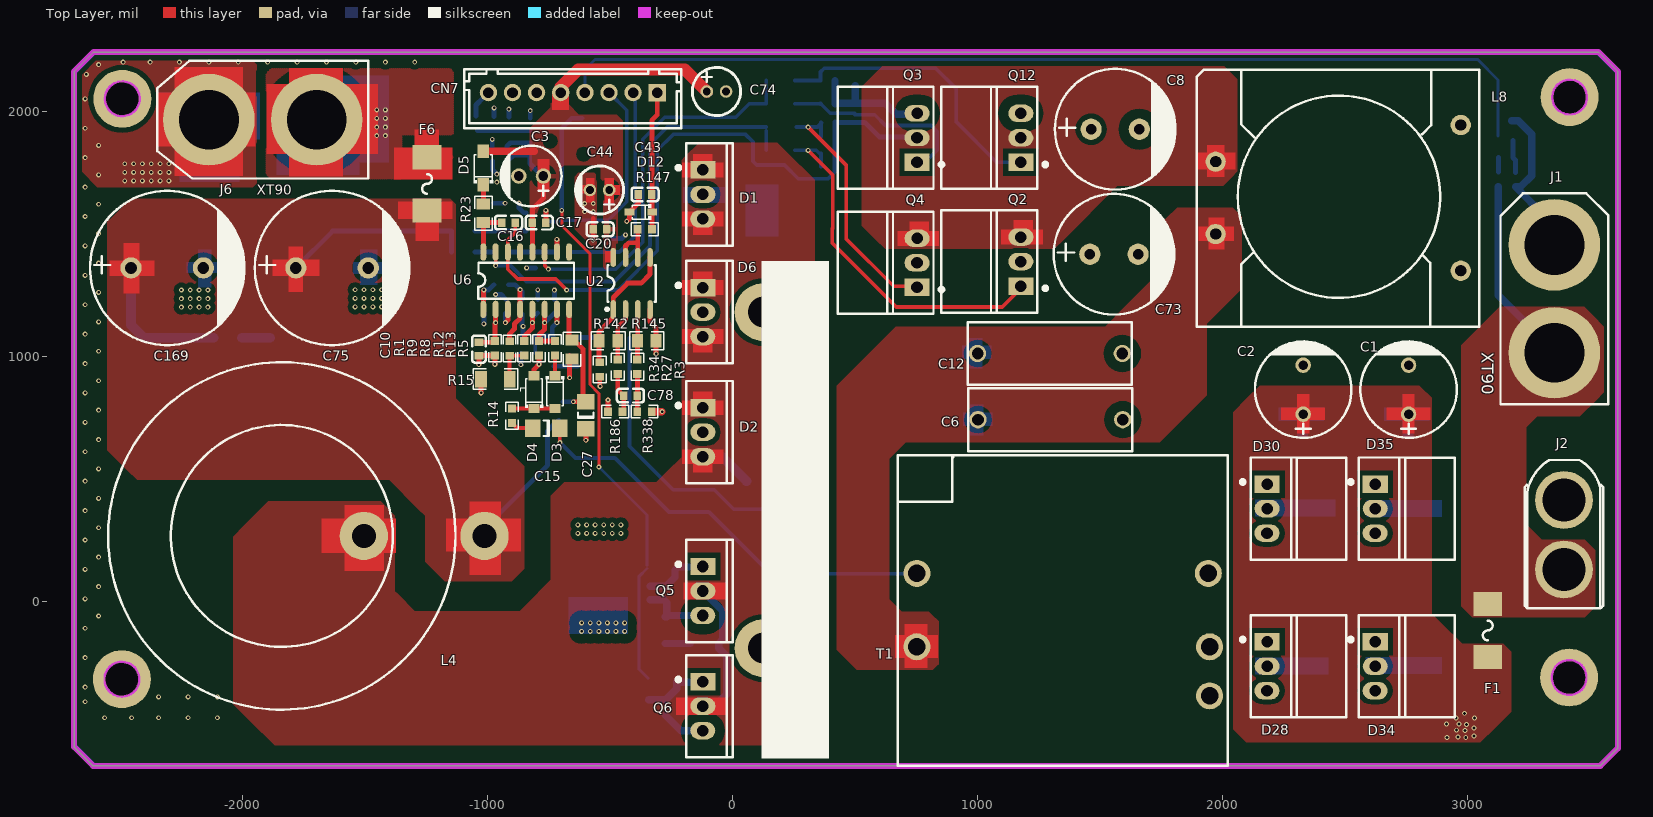
[diagram p0: Top Layer view]
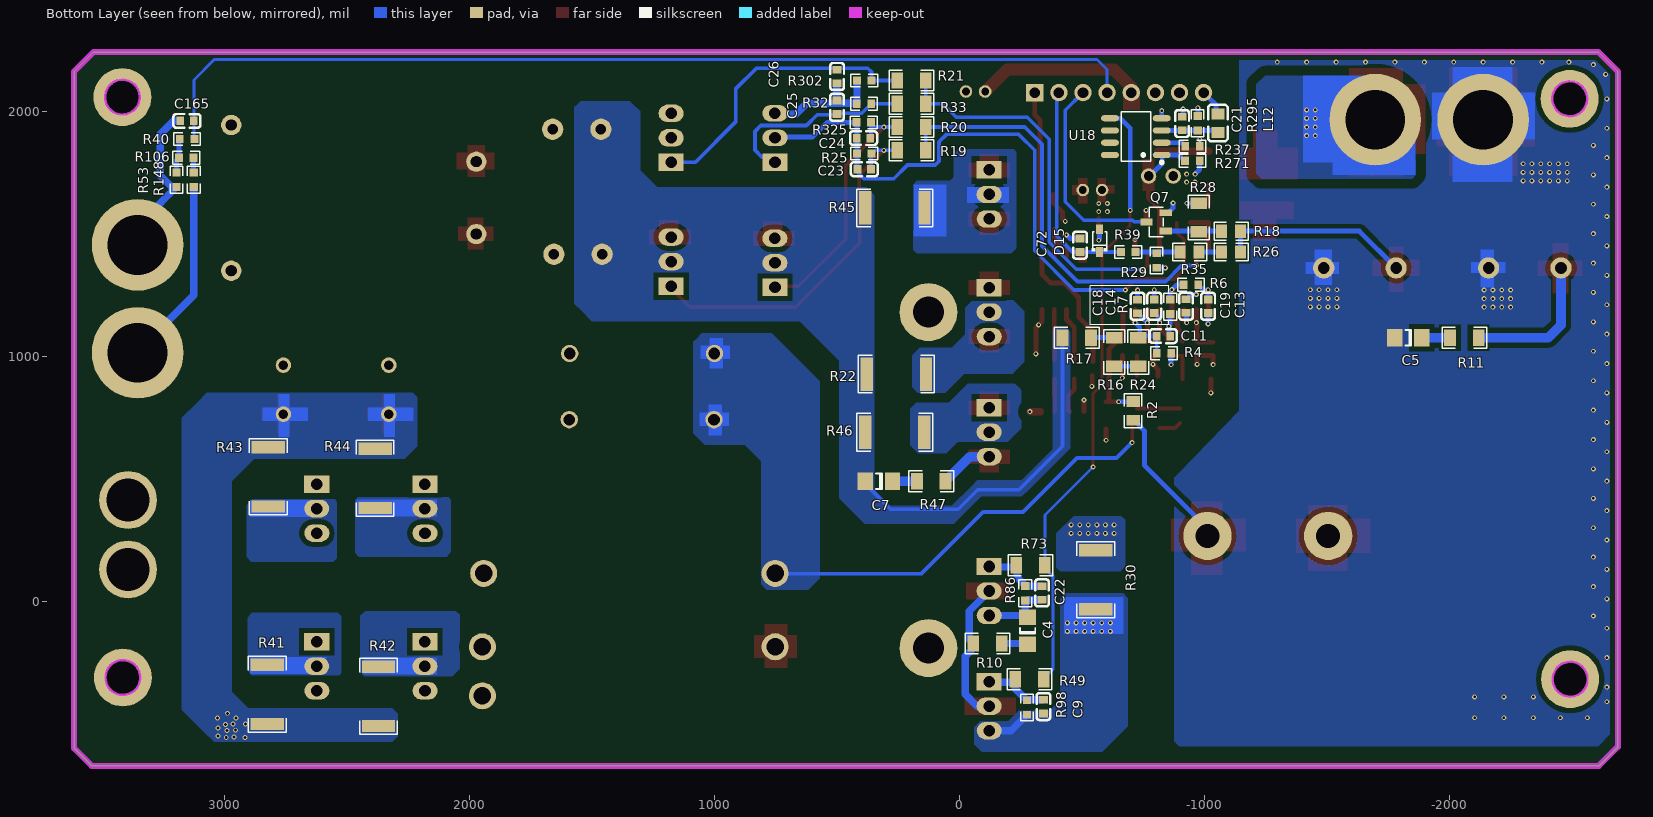
[diagram p1: Bottom Layer view, seen from below]
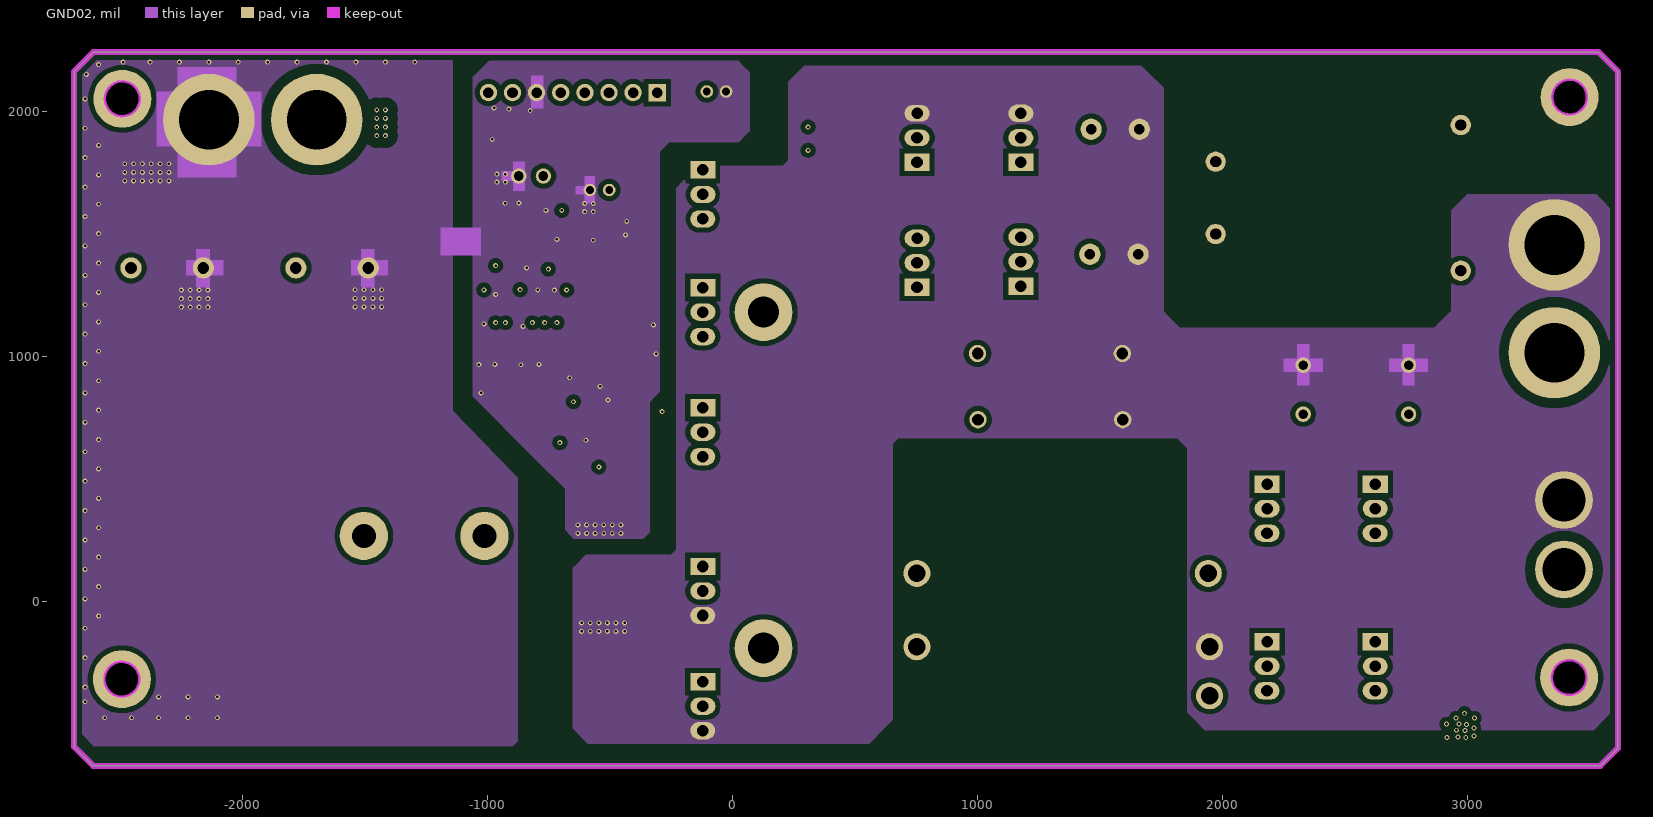
[diagram p2: GND02]
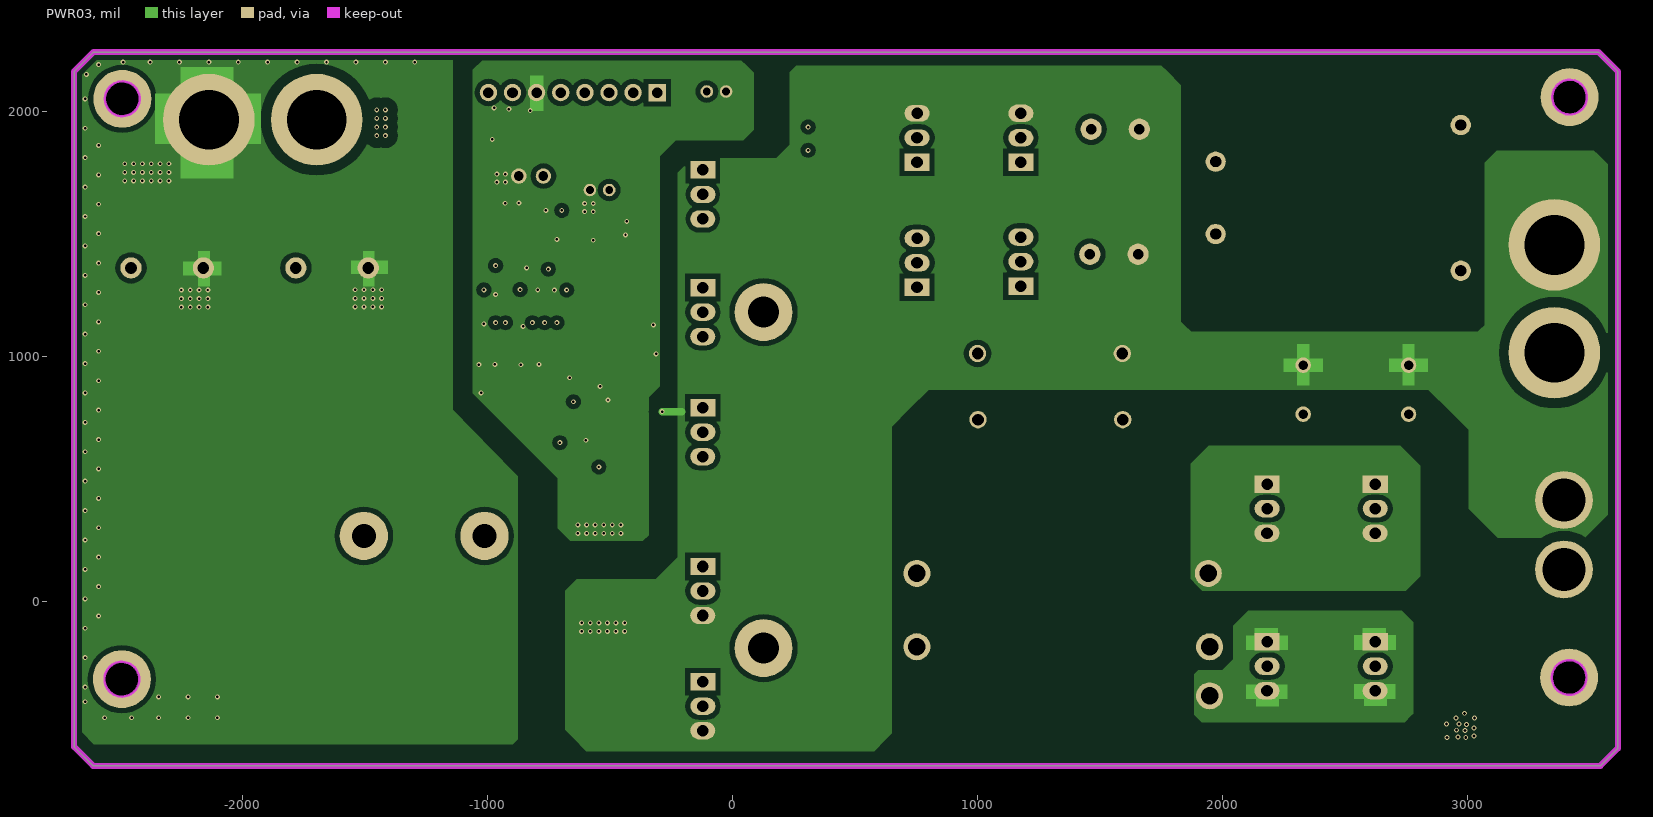
[diagram p3: PWR03]
# Altium PCB MISC89356.PcbDoc (part 1 of 3)
Units mil, origin at the board's own origin, x right, y up, seen from the top; angles counter-clockwise.
Board outline 6299.21 x 2912.91 mil, 4 copper layers (Top Layer, GND02, PWR03, Bottom Layer); 128 components, 68 nets, 313 pads, 200 vias.

## Layer stack, top to bottom (the 12.6 mil dielectric is the usual default, probably not edited)
Top Layer: signal copper 1.4
Dielectric: core 12.6, FR-4, Dk 4.8
GND02: signal copper 1.4
Dielectric: prepreg 12.6, FR-4, Dk 4.8
PWR03: signal copper 1.4
Dielectric: core 12.6, FR-4, Dk 4.8
Bottom Layer: signal copper 1.4

## Board outline
-2687.15,-592 -2609.15,-670 3539.85,-670 3612.07,-597.79 3612.07,2164.17 3533.33,2242.91 -2608.41,2242.91 -2687.15,2164.17

## Design rules (kind name [scope] priority, off if disabled: settings)
Clearance inpoly&Net [inpoly vs InNet('BAT-') or InNet('B+') or InNet('PV+')  or InNet('SW-PV') OR InNet('NETC75_1')] p1: gap=40
Clearance inpoly&inpoly [inpoly vs inpoly] p2: gap=20
Clearance INPOLY*All [INPOLY] p3: gap=20
Clearance Clearance_2 [isvia vs inpoly] p4: gap=10
Clearance Clearance_1 [All] p5: gap=8
ComponentClearance [All] p1 off: gap=10 collisioncheckmode=3 verticalgap=10 showdistances=FALSE
FabricationTestPointUsage TestPointUsage [All] p1: valid=0 allowmultiple=FALSE
FabricationTestpoint Testpoint [(IsPad And (OnTopLayer Or OnBottomLayer))] p1: side=3 testpointundercomponent=TRUE minsize=40 maxsize=100 preferedsize=60 minholesize=0 maxholesize=40 preferedholesize=32 testpointgrid=1 allowsidetop=TRUE allowsidebottom=TRUE usegrid=TRUE gridtolerance=0.01
Height [All] p1 off: minheight=0 maxheight=1000 prefheight=500
HoleSize [All] p1 off: absolutevalues=TRUE maxlimit=100 minlimit=1 maxpercent=80.000 minpercent=20.000
HoleToHoleClearance [All] p1 off: gap=10 allowstackedmicrovias=TRUE
LayerPairs [All] p1 off: enforce=TRUE
MinimumSolderMaskSliver [All] p1 off: minsoldermaskwidth=10
NetAntennae [All] p1: netantennaetolerance=1
PlaneClearance [All] p1: clearance=12
PlaneConnect [All] p1: planeconnectstyle=Relief reliefexpansion=8 reliefentries=4 reliefconductorwidth=10 reliefairgap=10
PolygonConnect PolygonConnect_1 [ISVIA] p1: connectstyle=Direct reliefconductorwidth=10 reliefentries=4 polygonreliefangle="90 Angle"
PolygonConnect [All] p2: connectstyle=Direct reliefconductorwidth=20 reliefentries=4 polygonreliefangle="90 Angle"
RoutingVias [All] p1: holewidth=10 width=20 viastyle="Through Hole" minholewidth=10 minwidth=20 maxholewidth=10 maxwidth=20
SilkToSilkClearance [All] p1 off: silktosilkclearance=10
SilkscreenOverComponentPads [IsPad] p1 off: minsilkscreentomaskgap=10
SolderMaskExpansion [All] p1: expansion=2.5
Width [All] p1: maxlimit=500 minlimit=10 preferedwidth=10
15 further rules are at their usual default settings.

## Components (designator, comment, footprint, x,y, rotation, side; value= is the part's Value field where it differs from the comment)
C1 "390uF" CAP-TH_BD10.0-P5.00-D1.0-FD 2757.85,867 r90 top
C2 "390uF" CAP-TH_BD10.0-P5.00-D1.0-FD 2327.85,867 r90 top
C3 "220uF" CAP-TH_BD6.3-P2.50-D1.0-FD -822.54,1737 r180 top
C4 "2.2nF" C1206 -278.15,-118.12 r90 bottom
C5 "2.2nF" C1206 -1832.03,1077 r0 bottom
C6 "150nF" CAP-TH_L17.0-W6.5-P15.00-D1.2 1296.41,743 r0 top
C7 "2.2nF" C1206 327.97,492 r0 bottom
C8 "150uF" CAP-TH_BD12.5-P5.00-D0.6-FD 1560.85,1928 r0 top
C9 "2.2nF" C0603 -343,-427.85 r270 bottom
C10 "220nF" C0603 -1035.15,1031.25 r90 top
C11 "1uF" C0603 -832.59,1083.69 r180 bottom
C12 "150nF" CAP-TH_L17.0-W6.5-P15.00-D1.2 1294.56,1013 r0 top
C13 "2.2uF" C0603 -1015.15,1206.14 r90 bottom
C14 "2.2uF" C0603 -795.15,1206.14 r270 bottom
C15 "NC" C1206 -760.03,708.69 r180 top
C16 "100nF" C0603 -914.59,1547 r180 top
C17 "100nF" C0603 -789.59,1547 r180 top
C18 "470pF" C0603 -727.15,1205.25 r270 bottom
C19 "1nF" C0603 -925.15,1206.25 r90 bottom
C20 "100nF" C0603 -541.27,1520 r180 top
C21 "220pF" C0603 -908.85,1951 r270 bottom
C22 "2.2nF" C0603 -337.15,36 r270 bottom
C23 "2.2nF" C0603 388,1764.85 r0 bottom
C24 "2.2nF" C0603 391,1891.85 r0 bottom
C25 "2.2nF" C0603 499.15,2018 r90 bottom
C26 "2.2nF" C0603 498.85,2143 r270 bottom
C27 "10nF" C1206 -599.15,761 r90 top
C43 "1nF" C0603 -357.15,1662 r0 top
C44 "22uF" CAP-TH_BD5.0-P2.00-D0.8-FD -543.08,1680 r180 top
C72 "100nF" C0603 -492.15,1454.67 r270 bottom
C73 "150uF" CAP-TH_BD12.5-P5.00-D0.6-FD 1555.85,1418 r0 top
C74 "22uF" CAP-TH_BD5.0-P2.00-D0.8-FD -66.15,2082 r0 top
C75 "560uF" CAP-TH_BD16.0-P7.50-D1.2-FD -1634.49,1362 r0 top
C78 "100nF" C0603 -416.83,841.01 r0 top
C165 "100nF" C0603 3151.41,1962 r180 bottom
C169 "560uF" CAP-TH_BD16.0-P7.50-D1.2-FD -2307.15,1362 r0 top
CN7 "HX25003-8A" CONN-TH_8P-P2.50_HX25003-8A -652.15,2052 r0 top
D1 "SBD20C200T" TO-220-3_L10.0-W4.5-P2.54-L -112.15,1662 r270 top
D2 "SBD20C200T" TO-220-3_L10.0-W4.5-P2.54-L -112.15,692 r270 top
D3 "1N4148W_C388533" SOD-123_L2.8-W1.8-LS3.7-RD -725.15,855.32 r270 top
D4 "1N4148W_C388533" SOD-123_L2.8-W1.8-LS3.7-RD -810.15,855.32 r90 top
D5 "FR107_C2760867" SOD-123FL_L2.7-W1.8-LS3.8-RD -1017.15,1770.3 r90 top
D6 "SBD20C200T" TO-220-3_L10.0-W4.5-P2.54-L -112.15,1182 r270 top
D12 "MM3Z3V3_C123917" SOD-323_L1.8-W1.3-LS2.5-RD -374.88,1590 r180 top
D15 "MM3Z3V3_C123917" SOD-323_L1.8-W1.3-LS2.5-RD -572.15,1473.27 r90 bottom
D28 "SBD20C200T" TO-220-3_L10.0-W4.5-P2.54-L-N#1 2180.32,-263 r270 top
D30 "SBD20C200T" TO-220-3_L10.0-W4.5-P2.54-L-N#1 2180.32,380 r270 top
D34 "SBD20C200T" TO-220-3_L10.0-W4.5-P2.54-L-N#1 2621.62,-263 r270 top
D35 "SBD20C200T" TO-220-3_L10.0-W4.5-P2.54-L-N#1 2621.62,380 r270 top
F1 "20A/200V" FUSE-SMD_L6.1-W2.5 3080.85,-117 r90 top
F6 "10A/200V" FUSE-SMD_L6.1-W2.5 -1247.15,1705.27 r270 top
J1 "" XT90N 3352.85,1236.23 r270 top
J2 "XT60" CONN-TH_XT60UPB-F 3391.85,276 r270 top
J6 "10V-90V 400W 5.6A MAX" XT90 -1917.15,1967 r0 top
L4 "230uH" IND-TH_CS343090*2-W231K -1731.22,268.66 r0 top
L8 "6.3uH" PQ2620-N 2470.85,1648 r0 top
L12 "BLM21PG300SN1D" L0805 -1055,1952.15 r270 bottom
Q2 "IRF640NPBF" TO-220-3_L10.0-W4.5-P2.54-L-N#1 1175.99,1388 r90 top
Q3 "IRF640NPBF" TO-220-3_L10.0-W4.5-P2.54-L-N#2 752.38,1893 r90 top
Q4 "IRF640NPBF" TO-220-3_L10.0-W4.5-P2.54-L-N#1 752.38,1383 r90 top
Q5 "KNP9120A" TO-220-3_L10.0-W4.5-P2.54-L -112.15,44 r270 top
Q6 "KNP9120A" TO-220-3_L10.0-W4.5-P2.54-L -112.15,-426 r270 top
Q7 "MMBT3904" SOT-23-3_L2.9-W1.3-P1.90-LS2.4-BR -802.78,1549.71 r180 bottom
Q12 "IRF640NPBF" TO-220-3_L10.0-W4.5-P2.54-L-N#1 1175.85,1893 r90 top
R1 "1.5M" R0603 -970.15,1034.04 r90 top
R2 "" R0805 -709,790.15 r270 bottom
R3 "" R0603 -388.71,959.37 r270 top
R4 "" R0603 -834.69,1013.8 r0 bottom
R5 "" R0805 -655.15,1018.04 r90 top
R6 "3K" R0603 -944.8,1293.69 r180 bottom
R7 "" R0603 -860.15,1204.04 r270 bottom
R8 "" R0603 -849.85,1033.96 r90 top
R9 "3.65K" R0603 -910.15,1033.69 r270 top
R10 "" R1206#1 -83.71,-159.64 r180 bottom
R11 "" R1206#1 -2091.87,1066.49 r0 bottom
R12 "" R0603 -790.15,1034.04 r90 top
R13 "" R0603 -725.15,1034.04 r90 top
R14 "" R0603 -900.15,759.04 r90 top
R15 "10K" R1206#1 -936.86,898.18 r180 top
R16 "" R1206#1 -642.65,1050.89 r270 bottom
R17 "" R1206#1 -447.42,1087.51 r180 bottom
R18 "100K" R0805 -1097.15,1512 r180 bottom
R19 "10" R1206#2 194.63,1842 r0 bottom
R20 "10" R1206#1 163.13,1926.49 r0 bottom
R21 "10" R1206#1 163.13,2116.49 r0 bottom
R22 "" R2512 256.57,929 r0 bottom
R23 "" R0805 -1017.15,1573.71 r90 top
R24 "33K" R1206#1 -719.64,987.88 r90 bottom
R25 "30K" R0603 388.2,1829 r0 bottom
R26 "100K" R0805 -1097.15,1427 r180 bottom
R27 "" R0603 -468.71,959.37 r270 top
R28 "10K" R1206#1 -965.85,1536.32 r90 bottom
R29 "2K" R0603 -804.85,1392.26 r270 bottom
R30 "" R2512 -556.15,89.72 r270 bottom
R32 "30K" R0603 388.89,2032 r0 bottom
R33 "10" R1206#2 194.63,2032 r0 bottom
R34 "1K" R0603 -542.15,947.35 r270 top
R35 "0" R0805 -927.77,1427.11 r180 bottom
R39 "" R0603 -689.23,1426.89 r0 bottom
R40 "" R0603 3150.86,1888 r0 bottom
R41 "" R2512 2823.85,-377.72 r270 bottom
R42 "" R2512 2369.85,-386 r270 bottom
R43 "" R2512 2819.85,509.28 r90 bottom
R44 "" R2512 2383.85,503.28 r90 bottom
R45 "" R2512 262.85,1607 r0 bottom
R46 "" R2512 263.57,692 r0 bottom
R47 "" R1206#1 83.13,481.49 r0 bottom
R49 "10" R1206#1 -318.2,-327 r0 bottom
R53 "30K" R0603 3193.85,1722.35 r90 bottom
R73 "10" R1206#1 -321.2,138 r0 bottom
R86 "30K" R0603 -269.15,34.35 r90 bottom
R98 "30K" R0603 -276.15,-431 r90 bottom
R106 "120K" R0603 3154.2,1812 r180 bottom
R142 "100K" R0805 -518.09,1065 r0 top
R145 "100K" R0805 -362,1065 r0 top
R147 "1K" R0603 -359.06,1520 r0 top
R148 "560K" R0603 3123.85,1722.35 r270 bottom
R186 "1" R0603 -478.93,776.01 r180 top
R237 "" R0603 -951.15,1858 r0 bottom
R271 "" R0603 -950.85,1799 r0 bottom
R295 "NC" R0603 -972.15,1952 r90 bottom
R302 "30K" R0603 388.2,2127 r0 bottom
R325 "30K" R0603 389.89,1956 r0 bottom
R338 "1" R0603 -359.62,776.01 r0 top
T1 "" "PQ3230 3:2:2-N" 1348.85,-134 r270 top locked
U2 "EG358" SOIC-8_L5.0-W4.0-P1.27-LS6.0-BL -385.16,1255.89 r0 top
U6 "EG6599" SO-16_L10.0-W4.0-P1.27-LS6.2-BL -842.21,1302.28 r0 top
U18 "EG3113" SOP-8_L4.9-W3.9-P1.27-LS6.0-BL -720.15,1898 r90 bottom

## Footprints (in the part's own frame and the unit in brackets; to place one, negate y for a bottom-side part, rotate by r counter-clockwise, add the part's x,y. Pads: shape width x height; smd on the part's side, far side on the other; paste and mask are expansions set on the pad)
C0603 [mm]
  rect 0.8x0.9 smd: 1(-0.7,0) 2(0.7,0)
  silkscreen extent -1.41,-0.71 1.39,0.72
C1206 [mm] "Chip Capacitor; Body 3.2 x 1.6 mm (LxW typ)"
  rect 1.6x1.8 smd: 1(-1.4,0) 2(1.4,0)
  silkscreen extent -0.3,-0.8 0.3,0.8
CAP-TH_BD5.0-P2.00-D0.8-FD [mm]
  round 1.3 hole 0.8: 1(-1,0) 2(1,0)
  silkscreen extent -2.5,-2.5 2.51,2.5
CAP-TH_BD6.3-P2.50-D1.0-FD [mm]
  round 1.6 hole 1: 1(-1.28,0) 2(1.26,0)
  silkscreen extent -3.16,-3.15 3.17,3.15
CAP-TH_BD10.0-P5.00-D1.0-FD [mm]
  round 1.6 hole 1: 1(-2.578,0) 2(2.502,0)
  silkscreen extent -5.04,-5 5.04,5
CAP-TH_BD12.5-P5.00-D0.6-FD [mm]
  round 2.2 hole 1.1: 1(-2.5,0) 2(2.5,0)
  silkscreen extent -6.25,-6.25 6.26,6.25
CAP-TH_BD16.0-P7.50-D1.2-FD [mm]
  round 2.2 hole 1.2: 1(-3.751,0) 2(3.749,0)
  silkscreen extent -8,-8 8.01,8
CAP-TH_L17.0-W6.5-P15.00-D1.2 [mm]
  round 1.8 hole 1.2: 1(-7.501,0) 2(7.501,0)
  silkscreen extent -8.5,-3.25 8.5,3.25
CONN-TH_8P-P2.50_HX25003-8A [mm]
  rect 1.8x1.8 hole 1.1: 1(8.75,0.646)
  round 1.8 hole 1.1: 2(6.25,0.646) 3(3.75,0.646) 4(1.25,0.646) 5(-1.25,0.646) 6(-3.75,0.646) 7(-6.25,0.646) 8(-8.75,0.646)
  silkscreen extent -11.25,-3.05 11.25,3.05
CONN-TH_XT60UPB-F [mm]
  round 6 hole 4.5: 1(3.663,0) 2(-3.536,0)
  silkscreen extent -7.68,-4.06 7.68,4.06
FUSE-SMD_L6.1-W2.5 [mm]
  rect 2.5x3 smd: 1(-2.75,0) 2(2.75,0)
  silkscreen extent -1.02,-0.51 1.02,0.51
IND-TH_CS343090*2-W231K [mm]
  round 5 hole 2.5: 1(18.25,0) 2(5.75,0)
  silkscreen extent -20.75,-18 15.25,18
L0805 [mil]
  rect 44.59x54.21 smd: 1(-38.05,0) 2(38.04,0)
  silkscreen extent -77,-40 73,40
PQ2620-N [mm]
  round 2.1 hole 1.1 slot 1.155 at 0 deg: 3(-12.7,3.75) 4(-12.7,-3.75) 8(12.7,-7.55) 11(12.7,7.55)
  silkscreen extent -14.68,-13.36 14.6,13.27
"PQ3230 3:2:2-N" [mm]
  round 2.8 hole 1.8: 3(-6.342,-15.17) 4(1.258,-15.17) 8(6.342,15.17) 9(1.262,15.17) 10(-6.342,15.03)
  silkscreen extent -18.59,-17.17 13.61,17.03
R0603 [mil]
  rect 31.75x34.02 smd: 1(-29.65,0) 2(29.65,0)
  silkscreen extent -55,-26 55,26
R0805 [mil]
  rect 44.59x54.21 smd: 1(-26.71,0) 2(49.37,0)
  silkscreen extent -58,-36 81,36
R1206#1 [mil]
  rect 47.54x66.97 smd: 1(-26.71,-10.51) 2(89.73,-10.51)
  silkscreen extent -59,-53 122,32
R1206#2 [mil]
  rect 47.54x66.97 smd: 1(-58.22,0) 2(58.22,0)
  silkscreen extent -91,-42 91,42
R2512 [mil]
  rect 50.49x136.06 smd: 1(-120.72,0) 2(120.72,0)
  silkscreen extent -155,-77 155,77
SO-16_L10.0-W4.0-P1.27-LS6.2-BL [mm]
  oval 0.6x1.8 smd: 1(-4.444,-2.776) 2(-3.174,-2.776) 3(-1.904,-2.776) 4(-0.634,-2.776) 5(0.636,-2.776) 6(1.906,-2.776) 7(3.176,-2.776) 8(4.446,-2.776) 9(4.446,3.168) 10(3.176,3.168) 11(1.906,3.168) 12(0.636,3.168) 13(-0.634,3.168) 14(-1.904,3.168) 15(-3.174,3.168) 16(-4.444,3.168)
  silkscreen extent -4.95,-1.65 4.95,2.05
SOD-123_L2.8-W1.8-LS3.7-RD [mm]
  rect 0.95x1.15 smd: 1(-1.693,0) 2(1.693,0)
  silkscreen extent -1.63,-0.94 1.41,0.94
SOD-123FL_L2.7-W1.8-LS3.8-RD [mm]
  rect 1.4x1.2 smd: 1(-1.735,0) 2(1.735,0)
  silkscreen extent -1.6,-1 1.38,1
SOD-323_L1.8-W1.3-LS2.5-RD [mm]
  rect 1x0.75 smd: 1(-1.173,0) 2(1.173,0)
  silkscreen extent -1.08,-0.8 0.9,0.8
SOIC-8_L5.0-W4.0-P1.27-LS6.0-BL [mil]
  oval 22.38x76.78 smd: 1(-101.98,-63.89) 2(-51.98,-63.89) 3(-1.98,-63.89) 4(48.02,-63.89) 5(48.02,149.11) 6(-1.98,149.11) 7(-51.98,149.11) 8(-101.98,149.11)
  silkscreen extent -133,-68 71,118
SOP-8_L4.9-W3.9-P1.27-LS6.0-BL [mm]
  oval 0.63x1.865 smd: 1(-1.905,-2.682) 2(-0.635,-2.682) 3(0.635,-2.682) 4(1.905,-2.682) 5(1.905,2.682) 6(0.635,2.682) 7(-0.635,2.682) 8(-1.905,2.682)
  silkscreen extent -2.82,-2.83 2.58,1.52
SOT-23-3_L2.9-W1.3-P1.90-LS2.4-BR [mm]
  rect 1.25x0.7 smd: 1(1,-0.95) 2(1,0.95) 3(-1,0)
  silkscreen extent -0.73,-1.53 0.73,1.53
TO-220-3_L10.0-W4.5-P2.54-L [mm]
  rect 1.8x2.6 hole 1.2: 1(-2.54,-0.241)
  oval 1.8x2.6 hole 1.2: 2(0,-0.241) 3(2.54,-0.251)
  silkscreen extent -5.3,-2.98 5.3,2.85
TO-220-3_L10.0-W4.5-P2.54-L-N#1 [mm]
  rect 1.8x2.6 hole 1.2: 1(-2.54,0.005)
  oval 1.8x2.6 hole 1.2: 2(0,0.005) 3(2.54,-0.005)
  silkscreen extent -5.3,-2.73 5.3,8.23
TO-220-3_L10.0-W4.5-P2.54-L-N#2 [mm]
  rect 1.8x2.6 hole 1.2: 1(-2.54,0.005)
  oval 1.727x2.6 hole 1.2: 2(0,0.005) 3(2.54,-0.005)
  silkscreen extent -5.3,-2.73 5.3,8.23
XT90 [mm]
  round 9.5 hole 6.2: 1(5.588,0) 2(-5.588,0)
  silkscreen extent -10.92,-6.1 10.92,6.1
XT90N [mm]
  round 9.5 hole 6.2: 1(5.588,0) 2(-5.588,0)
  silkscreen extent -10.92,-5.59 10.92,5.59

## Free pads (board coordinates)
  round 236.22 hole 141.73: 0(-2492.15,-315.95) 0(-2490.3,2052.2) 0(3412.93,-309.1) 0(3414.78,2059.05)
  round 236.22 hole 125.98: 0(125.98,-189.1) 0(125.98,1182)

## Via types
v1: diameter 20, hole 10, Top Layer to Bottom Layer, tented both sides, 177 vias
v2: diameter 20, hole 12, Top Layer to Bottom Layer, 13 vias
v3: diameter 20, hole 10, Top Layer to Bottom Layer, 10 vias

## Nets (pads, with @x,y where several pads share a name; then routed paths per layer and width w, separated by ;. In a path a pad name is that pad's centre, name@x,y a point inside that pad or via, vN(x,y) a via of type N, cw(c..) or ccw(c..) an arc to the next point about the centre after c; other vN are vias at no path point)
+12V: C3.1 C17.2 C20.1 C44.1 C74.1 CN7.5 D5.2 R271.2 U2.8 U6.12 U18.1 | length 1410
  Top Layer w20: U6.12@-817.15,1427 C17.2@-817.15,1547 -817.15,1602 -772.15,1647 C3.1@-772.15,1722
  Top Layer w30: D5.2@-1017.15,1838.61 -808.75,1838.61
  Top Layer w50: CN7.5@-701.35,2077.44 -701.35,2100.65 -630.08,2171.92 -195.44,2171.92 C74.1@-105.52,2082
  Bottom Layer w20: R271.2@-921.2,1799 -918,1799 -894,1823 U18.1@-841,1823 ; U18.1@-828,1823 -828,1788 -777,1737 C3.1@-772.15,1737
B+: F1.2 J1.1 J2.1 R148.2 | length 684.6
  Bottom Layer w30: R148.2@3123.85,1692.69 3123.85,1250.15 J1.1@3295,1079
BAT-: C1.2 C2.2 C4.2 C6.2 C8.2 C9.2 C12.2 C22.2 C25.2 C26.2 C73.2 C165.1 J1.2 J2.2 Q3.3 Q5.3 Q6.3 Q12.3 R30.2 R32.2 R53.1 R86.1 R98.1 R302.2 R338.2 T1.9 | length 1657.7
  Top Layer w30: R338.2@-329.97,776.01 v1(-288.14,776.01)
  PWR03 w30: v1(-288.14,776.01) -208.14,776.01
  Bottom Layer w30: C22.2@-337.15,8.44 -281.44,8.44 -269,-4 C4.2@-269,-33 ; R98.1@-276.15,-460.65 -210.8,-526 Q6.3@-121.01,-526 ; C4.2@-276.15,-61 -271.15,-56 C4.2@-269.15,-56 ; C4.2@-269.15,-61 C4.2@-269.15,-56 ; C4.2@-269.15,-33 C4.2@-269.15,-56 ; Q5.3@-121.01,-56 Q5.3@-122.01,-56 C4.2@-269.15,-56 ; R302.2@417.85,2127 417.85,2032.69 R32.2@418.54,2032 ; R32.2@425,2034 C25.2@500,2034 ; C26.2@500,2106 C25.2@500,2034 ; Q3.3@763,1989 668,1989 623,2034 C25.2@500,2034 ; C165.1@3178.96,1962 3206,1962 3260,1908 3260,1738 3214.69,1692.69 ; R53.1@3201,1692 3214,1692 3214.69,1692.69 ; J1.2@3314,1572.54 R53.1@3193.85,1692.69 3214.69,1692.69
  other v1: -616.15,-121 -581.15,-121 -546.15,-121 -511.15,-121 -476.15,-121 -441.15,-121 -616.15,-86 -581.15,-86 -546.15,-86 -511.15,-86 -476.15,-86 -441.15,-86
BAT-V: C165.2 CN7.4 R40.1 | length 4114.8
  Bottom Layer w12: CN7.4@-602.93,2077.44 -602.93,2171.22 -562.15,2212 2948,2212 ; 2962.85,2212 2948,2212 ; R40.1@3123,1900 3123,2129 3040,2212 2948,2212